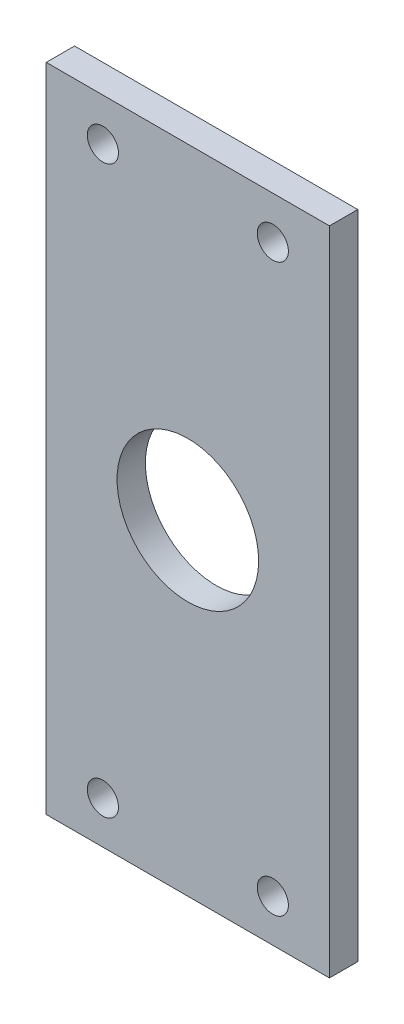
SolidWorks part; units mm, degrees
material "Q235B"
ref_plane "Front Plane" through (0, 0, 0) normal (0, 0, 1) x (1, 0, 0)
ref_plane "Top Plane" through (0, 0, 0) normal (0, 1, 0) x (1, 0, 0)
ref_plane "Right Plane" through (0, 0, 0) normal (1, 0, 0) x (0, 0, -1)
other "Configuration Table"
sketch "Sketch 1" plane through (0, 0, 0) normal (0, 0, 1) x (1, 0, 0)
  line L1 (-50, -115) -> (50, -115)
  line L2 (-50, -115) -> (-50, 115)
  line L3 (-50, 115) -> (50, 115)
  line L4 (50, -115) -> (50, 115)
  line L5 (-50, -115) -> (50, 115) construction
  line L6 (-50, 115) -> (50, -115) construction
  line L7 (-30, -100) -> (30, -100) construction
  line L8 (-30, -100) -> (-30, 100) construction
  line L9 (-30, 100) -> (30, 100) construction
  line L10 (30, -100) -> (30, 100) construction
  line L11 (-30, -100) -> (30, 100) construction
  line L12 (-30, 100) -> (30, -100) construction
  circle A0 centre (0, 0) radius 25
  circle A1 centre (-30, 100) radius 5.5
  circle A2 centre (30, 100) radius 5.5
  circle A3 centre (30, -100) radius 5.5
  circle A4 centre (-30, -100) radius 5.5
  point P0 (0, 0)
  point P6 (0, 0)
  dimension "D1" = 50
  dimension "D2" = 100
  dimension "D3" = 200
  dimension "D4" = 230
  dimension "D5" = 60
extrude "Boss-Extrude1" add sketch "Sketch 1" along normal blind 10
